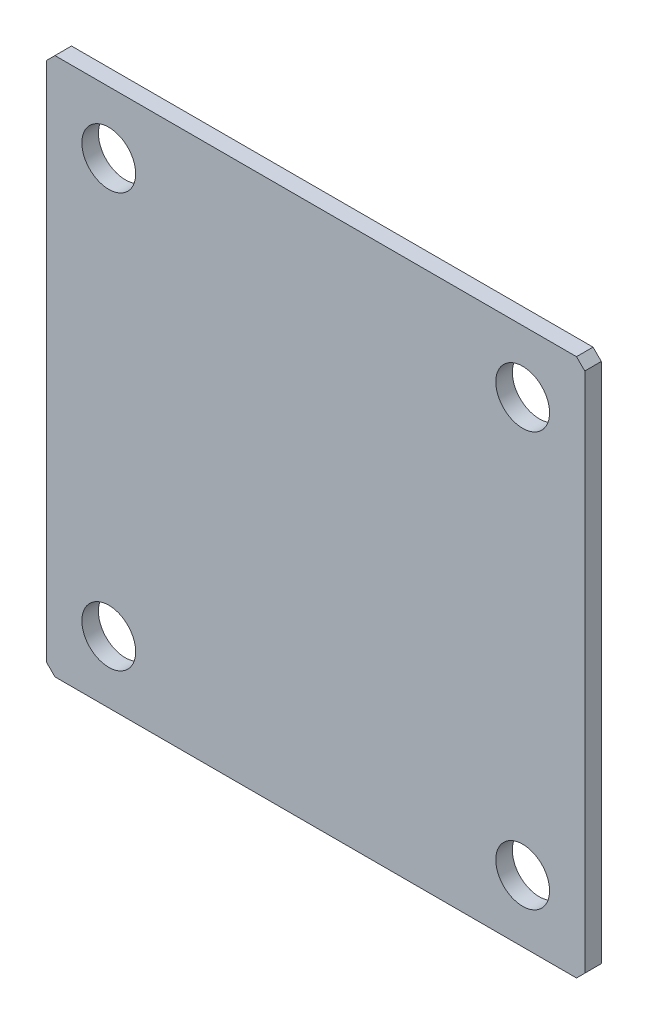
SolidWorks part; units mm, degrees
material "PF"
ref_plane "前基準面" through (0, 0, 0) normal (0, 0, 1) x (1, 0, 0)
ref_plane "上基準面" through (0, 0, 0) normal (0, 1, 0) x (1, 0, 0)
ref_plane "右基準面" through (0, 0, 0) normal (1, 0, 0) x (0, 0, -1)
sketch "草图1" plane through (0, 0, 0) normal (0, 0, 1) x (1, 0, 0)
  line L0 (0, 0) -> (-21.5083, 0) construction
  line L1 (0, 65) -> (-130, 65)
  line L2 (0, 65) -> (0, -65)
  line L3 (0, -65) -> (-130, -65)
  line L4 (-130, 65) -> (-130, -65)
  dimension "D1" = 130
  dimension "D2" = 130
extrude "凸台-拉伸1" add sketch "草图1" along normal blind 4
chamfer "倒角1" distance 2 angle 45 4 edges at (-130, 65, 2) (-130, -65, 2) (0, -65, 2) (0, 65, 2)
ref_plane "基准面1" through (-65, 0, 0) normal (-1, 0, 0) x (0, 0, 1)
hole_wizard "Ø13.0 (13) 直径孔1" positions "草图2" profile "草图3" hole size "Ø13.0" standard "GB" end condition through all
sketch "草图2" plane through (0, 0, 0) normal (0, 0, -1) x (-1, 0, 0)
  line L0 (0, 0) -> (130, 0) construction
  line L1 (130, 63) -> (130, -63) construction
  line L3 (115, -50) -> (15, -50) construction
  line L4 (115, -50) -> (115, 50) construction
  line L5 (115, 50) -> (15, 50) construction
  line L6 (15, -50) -> (15, 50) construction
  line L7 (65, 50) -> (65, -50) construction
  line L8 (115, 0) -> (15, 0) construction
  line L9 (65, -65) -> (65, 59.3987) construction
  line L10 (128, -65) -> (2, -65) construction
  point P10 (15, 50)
  point P203 (115, -50)
  point P204 (115, 50)
  point P205 (15, -50)
  dimension "D1" = 100
  dimension "D2" = 100
sketch "草图3" plane through (-15, -50, 0) normal (1, 0, 0) x (0, 1, 0)
  line L0 (0, 0) -> (0, 4)
  line L1 (0, 4) -> (6.5, 4)
  line L2 (6.5, 4) -> (6.5, 0)
  line L5 (6.5, 0) -> (0, 0)
  line L11 (0, -6.35) -> (0, 107.95) construction
  dimension "通孔孔直径" = 13
  dimension "通孔孔深度" = 4
